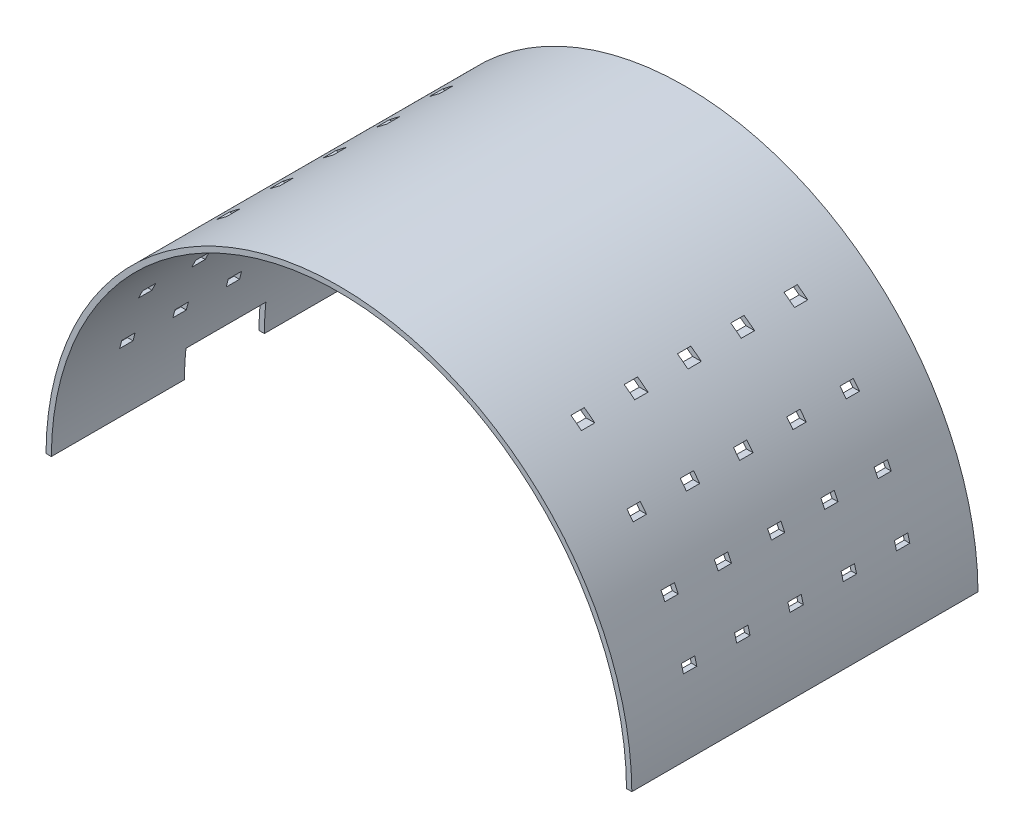
from build123d import *

# Parameters (mm, degrees)
EXTRUDE_1_DEPTH     = 130
SKETCH_2_W          = 10
SKETCH_2_H          = 6
CUT_EXTRUDE_1_DEPTH = 500
SKETCH_3_W          = 40
SKETCH_3_H          = 24
CUT_EXTRUDE_2_DEPTH = 30


with BuildPart() as part:
    # 草图1 → 凸台-拉伸1 (new, symmetric)
    with BuildSketch(Plane.XY):
        with BuildLine():
            Line((0.002272739, 1), (4.002314827, 1))
            ThreePointArc((4.002314827, 1), (220, 216), (435.997685173, 1))
            Line((435.997685173, 1), (439.997727261, 1))
            ThreePointArc((439.997727261, 1), (220, 220), (0.002272739, 1))
        make_face()
    extrude(amount=EXTRUDE_1_DEPTH, both=True)

    # 草图2 → 切除-拉伸1 (cut, symmetric)
    with BuildSketch(Plane(origin=(0, 0, 0), x_dir=(0, 0, -1), z_dir=(1, 0, 0))):
        with Locations((80, 55)):
            Rectangle(SKETCH_2_W, SKETCH_2_H)
        with Locations((40, 55)):
            Rectangle(SKETCH_2_W, SKETCH_2_H)
        with Locations((0, 55)):
            Rectangle(SKETCH_2_W, SKETCH_2_H)
        with Locations((-40, 55)):
            Rectangle(SKETCH_2_W, SKETCH_2_H)
        with Locations((-80, 55)):
            Rectangle(SKETCH_2_W, SKETCH_2_H)
        with Locations((80, 95)):
            Rectangle(SKETCH_2_W, SKETCH_2_H)
        with Locations((40, 95)):
            Rectangle(SKETCH_2_W, SKETCH_2_H)
        with Locations((0, 95)):
            Rectangle(SKETCH_2_W, SKETCH_2_H)
        with Locations((-40, 95)):
            Rectangle(SKETCH_2_W, SKETCH_2_H)
        with Locations((-80, 95)):
            Rectangle(SKETCH_2_W, SKETCH_2_H)
        with Locations((80, 135)):
            Rectangle(SKETCH_2_W, SKETCH_2_H)
        with Locations((40, 135)):
            Rectangle(SKETCH_2_W, SKETCH_2_H)
        with Locations((0, 135)):
            Rectangle(SKETCH_2_W, SKETCH_2_H)
        with Locations((-40, 135)):
            Rectangle(SKETCH_2_W, SKETCH_2_H)
        with Locations((-80, 135)):
            Rectangle(SKETCH_2_W, SKETCH_2_H)
        with Locations((80, 175)):
            Rectangle(SKETCH_2_W, SKETCH_2_H)
        with Locations((40, 175)):
            Rectangle(SKETCH_2_W, SKETCH_2_H)
        with Locations((0, 175)):
            Rectangle(SKETCH_2_W, SKETCH_2_H)
        with Locations((-40, 175)):
            Rectangle(SKETCH_2_W, SKETCH_2_H)
        with Locations((-80, 175)):
            Rectangle(SKETCH_2_W, SKETCH_2_H)
    extrude(amount=CUT_EXTRUDE_1_DEPTH, both=True, mode=Mode.SUBTRACT)

    # 草图3 → 切除-拉伸2 (cut, symmetric)
    with BuildSketch(Plane.XY):
        with Locations((10, 10)):
            Rectangle(SKETCH_3_W, SKETCH_3_H)
    extrude(amount=CUT_EXTRUDE_2_DEPTH, both=True, mode=Mode.SUBTRACT)


solid = part.part
